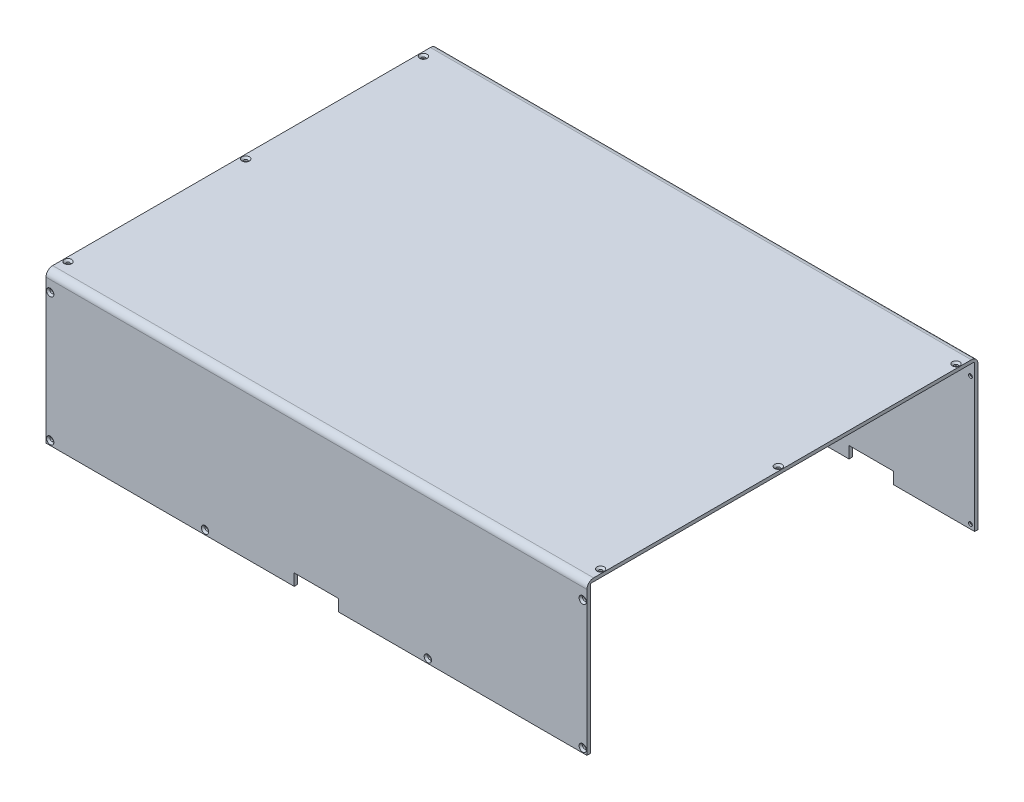
from build123d import *

# Parameters (mm, degrees)
SKETCH1_W                                       = 485.5
SKETCH1_H                                       = 132
BOSS_EXTRUDE1_DEPTH                             = 3
SKETCH2_W                                       = 485.5
SKETCH2_H                                       = 351
BOSS_EXTRUDE2_DEPTH                             = 3
SKETCH3_W                                       = 485.5
SKETCH3_H                                       = 3
BOSS_EXTRUDE3_DEPTH                             = 132
FILLET1_R                                       = 1
FILLET2_R                                       = 6
SKETCH4_W                                       = 40
SKETCH4_H                                       = 10.5
CUT_EXTRUDE1_DEPTH                              = 4.5
SKETCH5_W                                       = 40
SKETCH5_H                                       = 10.5
CUT_EXTRUDE2_DEPTH                              = 4.5
CROSS_RECESS_WOOD_SCREW_HOLE_TYPE_1_D           = 3.4
CROSS_RECESS_WOOD_SCREW_HOLE_TYPE_1_CSINK_D     = 6.6
CROSS_RECESS_WOOD_SCREW_HOLE_TYPE_1_CSINK_ANGLE = 90
CROSS_RECESS_WOOD_SCREW_HOLE_TYPE_2_D           = 3.4
CROSS_RECESS_WOOD_SCREW_HOLE_TYPE_2_DEPTH       = 6.5
CROSS_RECESS_WOOD_SCREW_HOLE_TYPE_2_CSINK_D     = 6.6
CROSS_RECESS_WOOD_SCREW_HOLE_TYPE_2_CSINK_ANGLE = 90
CROSS_RECESS_WOOD_SCREW_HOLE_TYPE_2_TIP         = 1.021463052
CROSS_RECESS_WOOD_SCREW_HOLE_TYPE_3_D           = 3.4
CROSS_RECESS_WOOD_SCREW_HOLE_TYPE_3_DEPTH       = 6.5
CROSS_RECESS_WOOD_SCREW_HOLE_TYPE_3_CSINK_D     = 6.6
CROSS_RECESS_WOOD_SCREW_HOLE_TYPE_3_CSINK_ANGLE = 90
CROSS_RECESS_WOOD_SCREW_HOLE_TYPE_3_TIP         = 1.021463052


with BuildPart() as part:
    # Sketch1 → Boss-Extrude1 (new body)
    with BuildSketch(Plane.XY):
        Rectangle(SKETCH1_W, SKETCH1_H)
    extrude(amount=BOSS_EXTRUDE1_DEPTH)

    # Sketch2 → Boss-Extrude2 (add)
    with BuildSketch(Plane(origin=(0, 66, 0), x_dir=(1, 0, 0), z_dir=(0, 1, 0))):
        with Locations((0, 172.5)):
            Rectangle(SKETCH2_W, SKETCH2_H)
    extrude(amount=BOSS_EXTRUDE2_DEPTH)

    # Sketch3 → Boss-Extrude3 (add)
    with BuildSketch(Plane.XZ.offset(-66)):
        with Locations((0, -346.5)):
            Rectangle(SKETCH3_W, SKETCH3_H)
    extrude(amount=BOSS_EXTRUDE3_DEPTH)

    # Fillet1
    fillet1_edges = [part.edges().sort_by_distance(p)[0] for p in [
        (0, 66, -345),
        (0, 66, 0),
    ]]
    fillet(fillet1_edges, radius=FILLET1_R)

    # Fillet2
    fillet2_edges = [part.edges().sort_by_distance(p)[0] for p in [
        (0, 69, 3),
        (0, 69, -348),
    ]]
    fillet(fillet2_edges, radius=FILLET2_R)

    # Sketch4 → Cut-Extrude1 (cut)
    with BuildSketch(Plane.XY.offset(3)):
        with Locations((0, -60.75)):
            Rectangle(SKETCH4_W, SKETCH4_H)
    extrude(amount=-CUT_EXTRUDE1_DEPTH, mode=Mode.SUBTRACT)

    # Sketch5 → Cut-Extrude2 (cut)
    with BuildSketch(Plane(origin=(0, 0, -348), x_dir=(-1, 0, 0), z_dir=(0, 0, -1))):
        with Locations((150, -60.75)):
            Rectangle(SKETCH5_W, SKETCH5_H)
        with Locations((-150, -60.75)):
            Rectangle(SKETCH5_W, SKETCH5_H)
    extrude(amount=-CUT_EXTRUDE2_DEPTH, mode=Mode.SUBTRACT)

    # Cross recess wood screw hole type 1 (through all)
    with Locations(Plane(origin=(0, 69, 0), x_dir=(1, 0, 0), z_dir=(0, 1, 0))):
        with Locations((239, 332), (239, 172.5), (239, 13), (-239, 332), (-239, 172.5), (-239, 13)):
            CounterSinkHole(CROSS_RECESS_WOOD_SCREW_HOLE_TYPE_1_D / 2, CROSS_RECESS_WOOD_SCREW_HOLE_TYPE_1_CSINK_D / 2, counter_sink_angle=CROSS_RECESS_WOOD_SCREW_HOLE_TYPE_1_CSINK_ANGLE)

    # Cross recess wood screw hole type 2
    with Locations(Plane.XY.offset(3)):
        with Locations((-239, 53), (-239, -62), (-100, -62), (100, -62), (239, 53), (239, -62)):
            CounterSinkHole(CROSS_RECESS_WOOD_SCREW_HOLE_TYPE_2_D / 2, CROSS_RECESS_WOOD_SCREW_HOLE_TYPE_2_CSINK_D / 2, depth=CROSS_RECESS_WOOD_SCREW_HOLE_TYPE_2_DEPTH, counter_sink_angle=CROSS_RECESS_WOOD_SCREW_HOLE_TYPE_2_CSINK_ANGLE)
            with Locations((0, 0, -(CROSS_RECESS_WOOD_SCREW_HOLE_TYPE_2_DEPTH + CROSS_RECESS_WOOD_SCREW_HOLE_TYPE_2_TIP / 2))):  # 118° drill point
                Cone(0, CROSS_RECESS_WOOD_SCREW_HOLE_TYPE_2_D / 2, CROSS_RECESS_WOOD_SCREW_HOLE_TYPE_2_TIP, mode=Mode.SUBTRACT)

    # Cross recess wood screw hole type 3
    with Locations(Plane(origin=(0, 0, -348), x_dir=(-1, 0, 0), z_dir=(0, 0, -1))):
        with Locations((239, 53), (239, -62), (100, -62), (-100, -62), (-239, -62), (-239, 53)):
            CounterSinkHole(CROSS_RECESS_WOOD_SCREW_HOLE_TYPE_3_D / 2, CROSS_RECESS_WOOD_SCREW_HOLE_TYPE_3_CSINK_D / 2, depth=CROSS_RECESS_WOOD_SCREW_HOLE_TYPE_3_DEPTH, counter_sink_angle=CROSS_RECESS_WOOD_SCREW_HOLE_TYPE_3_CSINK_ANGLE)
            with Locations((0, 0, -(CROSS_RECESS_WOOD_SCREW_HOLE_TYPE_3_DEPTH + CROSS_RECESS_WOOD_SCREW_HOLE_TYPE_3_TIP / 2))):  # 118° drill point
                Cone(0, CROSS_RECESS_WOOD_SCREW_HOLE_TYPE_3_D / 2, CROSS_RECESS_WOOD_SCREW_HOLE_TYPE_3_TIP, mode=Mode.SUBTRACT)


solid = part.part
